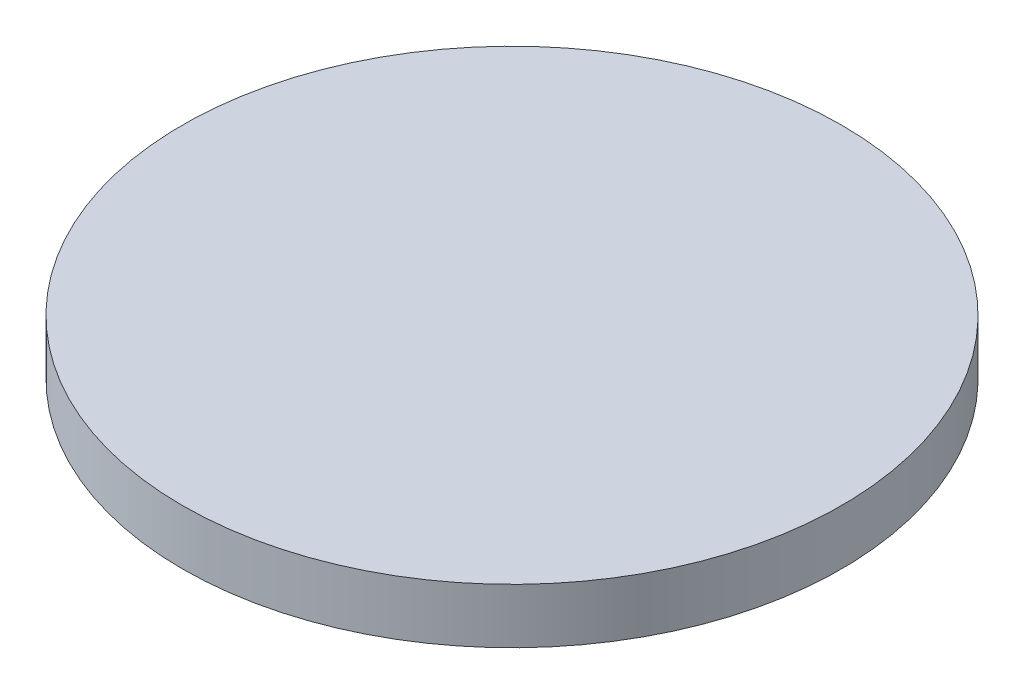
SolidWorks part; units mm, degrees
material "S45C"
ref_plane "Front Plane" through (0, 0, 0) normal (0, 0, 1) x (1, 0, 0)
ref_plane "Top Plane" through (0, 0, 0) normal (0, 1, 0) x (1, 0, 0)
ref_plane "Right Plane" through (0, 0, 0) normal (1, 0, 0) x (0, 0, -1)
sketch "Sketch1" plane through (0, 0, 0) normal (0, 1, 0) x (1, 0, 0)
  circle A0 centre (0, 0) radius 30
  dimension "D1" = 60
extrude "Boss-Extrude1" add sketch "Sketch1" along normal blind 5
